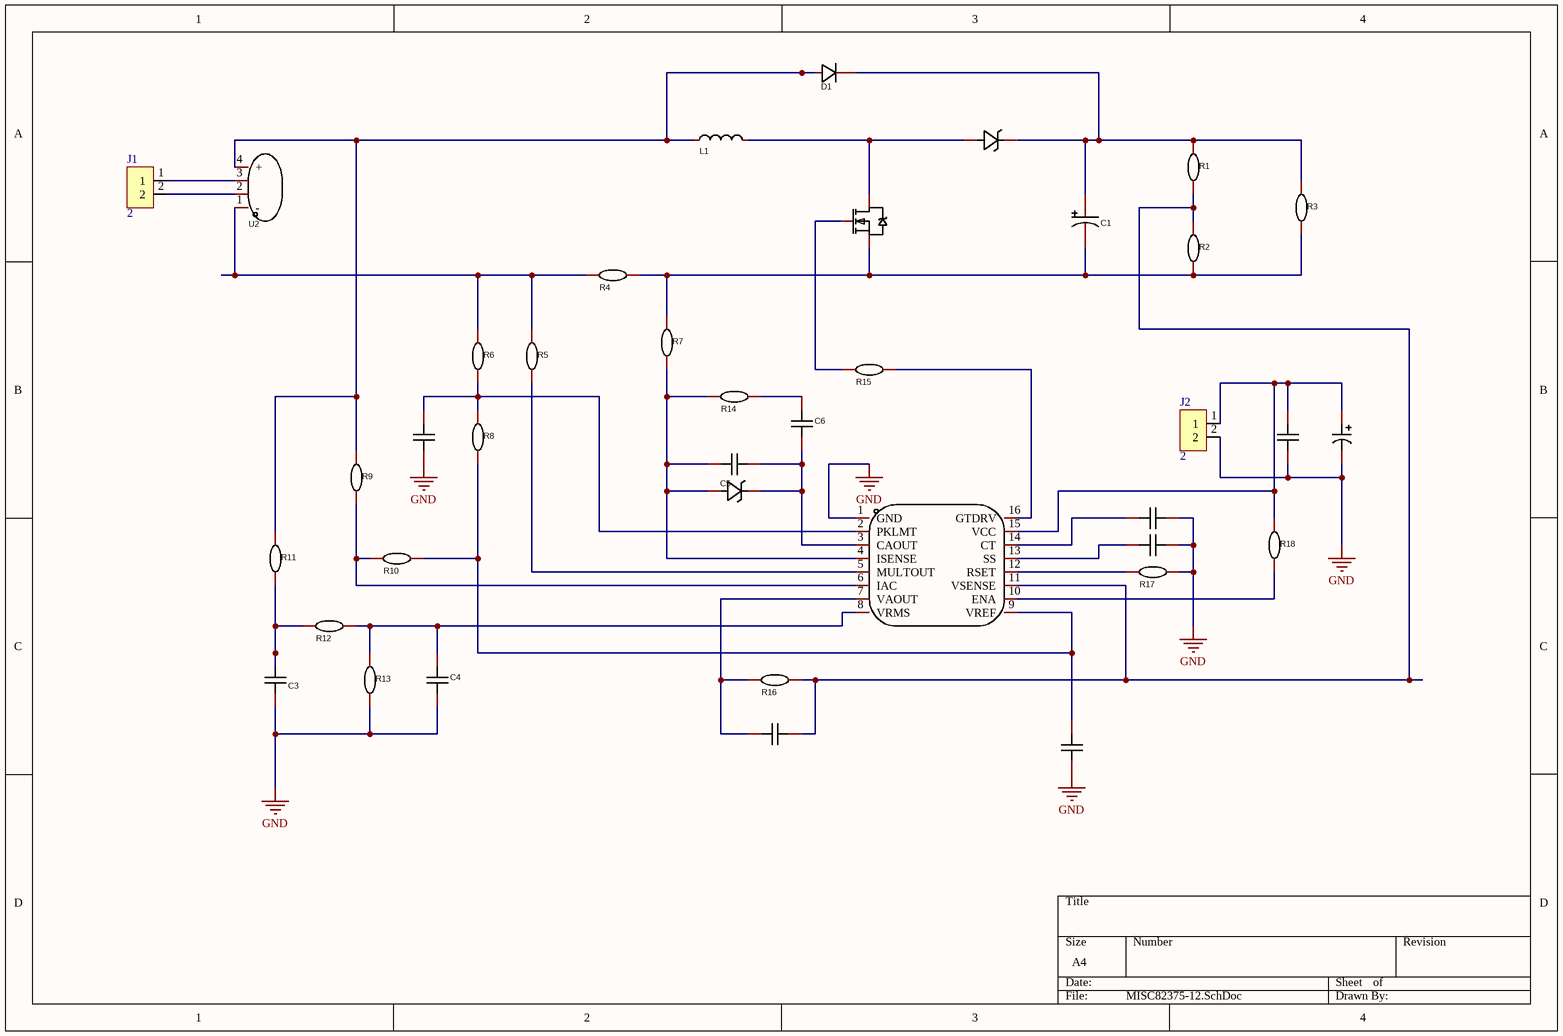
[diagram p0: MISC82375-12.SchDoc]
# Altium project MISC82375-12.PrjPcb
1 sheet, 39 parts. Net scope: global (net labels, ports and power ports of the same name join across sheets).
Board files: MISC82375-2.PcbDoc, MISC82375-4.PcbDoc, MISC82375-6.PcbDoc

## Sheet MISC82375-12.SchDoc
size A4; SheetNumber: 1; SheetTotal: 1

### Parts
C1  LKME1402A101MF  [CAP-TH_BD10.0-P5.00-D1.0-FD]  (value not drawn)
C2  KJKF222M2FF7035A075E  [CAP-TH_L6.5-W3.5-P7.50-D1.0]  (value not drawn)
C3  KY1102M400VAC70Y10093  [CAP-TH_L7.5-W4.5-P10.00-D0.6]  (value not drawn)
C4  CBB21-400V/255JP20  [CAP-TH_L22.0-W12.5-P20.00-D0.7-FD]  (value not drawn)
C5  178MU0002  [CAP-TH_L5.8-W3.6-P5.0-D0.6]  (value not drawn)
C6  178MU0002  [CAP-TH_L5.8-W3.6-P5.0-D0.6]  (value not drawn)
C7  KY1102M400VAC70Y10093  [CAP-TH_L7.5-W4.5-P10.00-D0.6]  (value not drawn)
C8  178MU0002  [CAP-TH_L5.8-W3.6-P5.0-D0.6]  (value not drawn)
C9  178MU0002  [CAP-TH_L5.8-W3.6-P5.0-D0.6]  (value not drawn)
C10  178MU0002  [CAP-TH_L5.8-W3.6-P5.0-D0.6]  (value not drawn)
C11  KY1102M400VAC70Y10093  [CAP-TH_L7.5-W4.5-P10.00-D0.6]  (value not drawn)
C??  RVE100UF35V67RV0072  [CAP-SMD_BD6.3-L6.6-W6.6-LS7.6-FD-1]  (value not drawn)
D1  1N5406_C5338388  [DO-27_BD5.2-L8.9-P12.90-D1.5-RD]  (value not drawn)
D2  GC3D10060A  [TO-220-2_L10.2-W4.5-P5.08-L-A]  (value not drawn)
D3  BZT52C8V2_C19077406  [SOD-123_L2.7-W1.6-LS3.7-RD]  (value not drawn)
J1  2  [DIP2 - duplicate]
J2  2  [DIP2 - duplicate]
L1  XR8*10-101K-L  [IND-TH_BD10.0-P5.00-D0.6]  (value not drawn)
Q1  IRF530NPBF  [TO-220-3_L10.0-W4.5-P2.54-L]  (value not drawn)
R1  MF1/4W-100K±1%-OT26  [RES-TH_BD2.7-L6.2-P10.20-D0.4]  (value not drawn)
R2  MF1/4W-100K±1%-OT26  [RES-TH_BD2.7-L6.2-P10.20-D0.4]  (value not drawn)
R3  MF1/4W-100K±1%-OT26  [RES-TH_BD2.7-L6.2-P10.20-D0.4]  (value not drawn)
R4  MF1/4W-100K±1%-OT26  [RES-TH_BD2.7-L6.2-P10.20-D0.4]  (value not drawn)
R5  MF1/4W-100K±1%-OT26  [RES-TH_BD2.7-L6.2-P10.20-D0.4]  (value not drawn)
R6  MF1/4W-100K±1%-OT26  [RES-TH_BD2.7-L6.2-P10.20-D0.4]  (value not drawn)
R7  MF1/4W-100K±1%-OT26  [RES-TH_BD2.7-L6.2-P10.20-D0.4]  (value not drawn)
R8  MF1/4W-100K±1%-OT26  [RES-TH_BD2.7-L6.2-P10.20-D0.4]  (value not drawn)
R9  MF1/4W-100K±1%-OT26  [RES-TH_BD2.7-L6.2-P10.20-D0.4]  (value not drawn)
R10  MF1/4W-100K±1%-OT26  [RES-TH_BD2.7-L6.2-P10.20-D0.4]  (value not drawn)
R11  MF1/4W-100K±1%-OT26  [RES-TH_BD2.7-L6.2-P10.20-D0.4]  (value not drawn)
R12  MF1/4W-100K±1%-OT26  [RES-TH_BD2.7-L6.2-P10.20-D0.4]  (value not drawn)
R13  MF1/4W-100K±1%-OT26  [RES-TH_BD2.7-L6.2-P10.20-D0.4]  (value not drawn)
R14  MF1/4W-100K±1%-OT26  [RES-TH_BD2.7-L6.2-P10.20-D0.4]  (value not drawn)
R15  MF1/4W-100K±1%-OT26  [RES-TH_BD2.7-L6.2-P10.20-D0.4]  (value not drawn)
R16  MF1/4W-100K±1%-OT26  [RES-TH_BD2.7-L6.2-P10.20-D0.4]  (value not drawn)
R17  MF1/4W-100K±1%-OT26  [RES-TH_BD2.7-L6.2-P10.20-D0.4]  (value not drawn)
R18  MF1/4W-100K±1%-OT26  [RES-TH_BD2.7-L6.2-P10.20-D0.4]  (value not drawn)
U1  UC3854N  [PDIP-16_L19.3-W6.4-P2.54-LS7.94-BL]  (value not drawn)
U2  GBU8K  [GBU_4P-L22.0-W3.5-P5.08-GBU4K]  (value not drawn)

### Nets
GND: C2.1 C3.1 C4.1 C8.1 C9.2 C10.2 C11.1 C??.2 J2.2 R13.1 R17.2 U1.1(GND)
NetC1_1: C1.1 D1.1(C) D2.1(K) R1.2 R3.2
NetC1_2: C1.2 Q1.3(S) R2.1 R3.1 R4.2 R7.2
NetC2_2: C2.2 R6.1 R8.2 U1.2(PKLMT)
NetC3_2: C3.2 R11.1 R12.1
NetC4_2: C4.2 R12.2 R13.2 U1.8(VRMS)
NetC5_1: C5.1 D3.2(A) R7.1 R14.1 U1.4(ISENSE)
NetC5_2: C5.2 C6.1 D3.1(K) U1.3(CAOUT)
NetC6_2: C6.2 R14.2
NetC7_1: C7.1 R16.1 U1.7(VAOUT)
NetC7_2: C7.2 R1.1 R2.2 R16.2 U1.11(VSENSE)
NetC8_2: C8.2 R8.1 R10.2 U1.9(VREF)
NetC9_1: C9.1 U1.13(SS)
NetC10_1: C10.1 U1.14(CT)
NetC11_2: C11.2 C??.1 J2.1 R18.2 U1.15(VCC)
NetD1_2: D1.2(A) L1.1 R9.2 R11.2 U2.4(+)
NetD2_3: D2.3(A) L1.2 Q1.2(D)
NetJ1_1: J1.1 U2.3
NetJ1_2: J1.2 U2.2
NetQ1_1: Q1.1(G) R15.1
NetR4_1: R4.1 R5.2 R6.2 U2.1(-)
NetR5_1: R5.1 U1.5(MULTOUT)
NetR9_1: R9.1 R10.1 U1.6(IAC)
NetR15_2: R15.2 U1.16(GTDRV)
NetR17_1: R17.1 U1.12(RSET)
NetR18_1: R18.1 U1.10(ENA)

### Library data of the parts
C1 = LKME1402A101MF: Manufacturer: Ymin(永铭); Add into BOM: yes; Value: 100uF; Tolerance: ±20%; Rated Voltage: 100V; Ripple Current: 1.04A@100kHz; φD: 10mm; L: 14mm; Lifetime @ Temp: 10000hrs@105℃; Symbol: LKME1402A101MF; Device: LKME1402A101MF; LCSC Part Name: 100uF ±20% 100V; Supplier Part: C443138; Manufacturer Part: LKME1402A101MF; Supplier Footprint: 插件,D10xL14mm; JLCPCB Part Class: Extended Part; Datasheet: https://atta.szlcsc.com/upload/public/pdf/source/20200220/C487520_443A40905984A455D375EE990FEAA9E8.pdf; Supplier: LCSC; Convert to PCB: yes; Equivalent Series Resistance(ESR): -; Lead Spacing: 5mm
C2 = KJKF222M2FF7035A075E: Manufacturer: KNSCHA(科尼盛); Add into BOM: yes; Value: 2.2nF; Tolerance: ±20%; Voltage(AC): 300V; Subclass: Y2; safety certification: UL; ENEC; VDE; CQC; Symbol: KJKF222M2FF7035A075E; Device: KJKF222M2FF7035A075E; LCSC Part Name: 2.2nF ±20% 300V 等级:Y2; Supplier Part: C2803195; Manufacturer Part: KJKF222M2FF7035A075E; Supplier Footprint: 插件,P=7.5mm; JLCPCB Part Class: Extended Part; Datasheet: https://atta.szlcsc.com/upload/public/pdf/source/20210420/C2803195_BA0DBC8778A43A5602C5594119034AD5.pdf; Supplier: LCSC; Convert to PCB: yes
C3 C7 C11 = KY1102M400VAC70Y10093: Manufacturer: KNSCHA(科尼盛); Value: 1nF; Add into BOM: yes; Tolerance: ±20%; Voltage(AC): 400V; Subclass: Y1; safety certification: UL; ENEC; VDE; CQC; Symbol: KY1102M400VAC70Y10093; Device: KY1102M400VAC70Y10093; Supplier: LCSC; Supplier Part: C2943996; Manufacturer Part: KY1102M400VAC70Y10093; JLCPCB Part Class: Extended Part; LCSC Part Name: 1nF ±20% 400V 等级:Y1; Supplier Footprint: 插件,P=10mm; Datasheet: https://atta.szlcsc.com/upload/public/pdf/source/20220125/2D2B80E2C5D988A5B116EA64517B63EA.pdf; Convert to PCB: yes
C4 = CBB21-400V/255JP20: Manufacturer: 东通电子; Add into BOM: yes; Value: 2.5uF; Tolerance: ±5%; Voltage Rated: 400V; Symbol: CBB21-400V/255JP20; Device: CBB21-400V/255JP20; LCSC Part Name: 2.5uF ±5% 400V; Supplier Part: C2913178; Manufacturer Part: CBB21-400V/255JP20; Supplier Footprint: 插件,P=20mm; JLCPCB Part Class: Extended Part; Datasheet: https://atta.szlcsc.com/upload/public/pdf/source/20211116/A54D0E5F37ACF7C4504A98327CA0E134.pdf; Supplier: LCSC; Convert to PCB: yes
C5 C6 C8-C10 = 178MU0002: Manufacturer: KNSCHA(科尼盛); Value: 100nF; Add into BOM: yes; Tolerance: ±10%; Voltage Rated: 50V; Temperature Coefficient: X7R; Symbol: 178MU0002; Device: 178MU0002; Supplier: LCSC; Supplier Part: C5632426; Manufacturer Part: 178MU0002; JLCPCB Part Class: Extended Part; LCSC Part Name: 100nF ±10% 50V; Supplier Footprint: 插件,P=5.08mm; Datasheet: https://atta.szlcsc.com/upload/public/pdf/source/20230506/08E784E6BF236BA57EBA91152AC3AC6D.pdf; Convert to PCB: yes
C?? = RVE100UF35V67RV0072: Manufacturer: KNSCHA(科尼盛); Add into BOM: yes; Value: 100uF; Tolerance: ±20%; Rated Voltage: 35V; Ripple Current: 230mA@120Hz; Equivalent Series Resistance(ESR): 600mΩ@100kHz; φD: 6.3mm; L: 7.7mm; Lifetime @ Temp: 2000hrs@105℃; Symbol: RVE100UF35V67RV0072; Device: RVE100UF35V67RV0072; LCSC Part Name: 100uF ±20% 35V; Supplier Part: C2836437; Manufacturer Part: RVE100UF35V67RV0072; Supplier Footprint: SMD,D6.3xL7.7mm; JLCPCB Part Class: Extended Part; Datasheet: https://atta.szlcsc.com/upload/public/pdf/source/20220719/B52EB46F8A1558448ED03D8B4CB3C24F.pdf; Supplier: LCSC; Convert to PCB: yes; Operating Temperature: -55℃~+105℃
D1 = 1N5406_C5338388: Manufacturer: SUNMATE(森美特); Manufacturer Part: 1N5406; Add into BOM: yes; Forward Voltage (Vf@If): 1V@3A; Reverse Voltage (Vr): 600V; Average Rectified Current (Io): 3A; Reverse Leakage Current: 10uA@600V; Symbol: 1N5406_C5338388; Device: 1N5406_C5338388; LCSC Part Name: 电压:600V 电流:3A; Supplier Part: C5338388; Supplier Footprint: DO-27; Datasheet: https://atta.szlcsc.com/upload/public/pdf/source/20221227/E8B5F2A8C1FD9CCCBF5FF47F6842D4A3.pdf; Supplier: LCSC; Convert to PCB: yes
D2 = GC3D10060A: Manufacturer: SUPSiC(国晶微半导体); Add into BOM: yes; Average Rectified Current (Io): 30A; Forward Voltage (Vf@If): 1.5V; Reverse Voltage (Vr): 600V; Symbol: GC3D10060A; Device: GC3D10060A; LCSC Part Name: GC3D10060A; Supplier Part: C7435067; Manufacturer Part: GC3D10060A; Supplier Footprint: TO-220-2; Datasheet: https://atta.szlcsc.com/upload/public/pdf/source/20230905/31DB1507024993D4A9FE1C88E19B495D.pdf; Supplier: LCSC; Convert to PCB: yes
D3 = BZT52C8V2_C19077406: Manufacturer: 宏迦橙; Add into BOM: yes; Diode Configuration: parameter Diode Configuration Single; Zener Voltage (Nom): 8.2V; Reverse Leakage Current (Ir): 700nA@5V; Zener Voltage (Range): 7.79V~8.61V; Power Dissipation: 500mW; Zener Impedance (Zzt): 15Ω; Symbol: BZT52C8V2_C19077406; Device: BZT52C8V2_C19077406; Supplier: LCSC; Supplier Part: C19077406; Manufacturer Part: BZT52C8V2; LCSC Part Name: BZT52C8V2; Supplier Footprint: SOD-123; Datasheet: https://atta.szlcsc.com/upload/public/pdf/source/20231117/6E01C14CCA1A38C68A5225952E4BCE14.pdf; Convert to PCB: yes
J1 J2 = AC_in
L1 = XR8*10-101K-L: Manufacturer: XR(祥如); Add into BOM: yes; Value: 100uH; Tolerance: ±10%; Type: parameter Type text I-type inductor; Symbol: XR8*10-101K-L; Device: XR8*10-101K-L; LCSC Part Name: 100uH ±10% 工字电感; Supplier Part: C5380241; Manufacturer Part: XR8*10-101K-L; Supplier Footprint: 插件,D8xL10mm; JLCPCB Part Class: Extended Part; Datasheet: https://atta.szlcsc.com/upload/public/pdf/source/20230323/E8473EC4B67CAA12E996DDE863677D9C.pdf; Supplier: LCSC; Convert to PCB: yes
Q1 = IRF530NPBF: Manufacturer: Infineon(英飞凌); Add into BOM: yes; Type: parameter Type text N-channel; Drain Source Voltage (Vdss): 100V; Continuous Drain Current (Id): 17A; Power Dissipation (Pd): 70W; Drain Source On Resistance (RDS(on)@Vgs,Id): 90mΩ@10V,9A; Gate Threshold Voltage (Vgs(th)@Id): 4V@250uA; Total Gate Charge (Qg@Vgs): 37nC@10V; Input Capacitance (Ciss@Vds): 920pF@25V; Symbol: IRF530NPBF; Device: IRF530NPBF; LCSC Part Name: N沟道 耐压:100V 电流:17A; Supplier Part: C2565; Manufacturer Part: IRF530NPBF; Supplier Footprint: TO-220AB; JLCPCB Part Class: Extended Part; Datasheet: https://atta.szlcsc.com/upload/public/pdf/source/20200421/C513195_D9CEFFCD00D3D7736B96C248E8CC28A6.pdf; Supplier: LCSC; Convert to PCB: yes; Operating Temperature: -55℃~+175℃@(Tj)
R1-R18 = MF1/4W-100K±1%-OT26: Manufacturer: VO(翔胜); Value: 100kΩ; Add into BOM: yes; Tolerance: ±1%; Overload Voltage (Max): 250V; Power(Watts): 250mW; Temperature Coefficient: ±350ppm/℃; Symbol: MF1/4W-100K±1%-OT26; Device: MF1/4W-100K±1%-OT26; Supplier: LCSC; Supplier Part: C2843019; Manufacturer Part: MF1/4W-100K±1%-OT26; JLCPCB Part Class: Extended Part; LCSC Part Name: 金属膜电阻 100kΩ ±1% 250mW; Supplier Footprint: 插件,2.7x6.2mm; Datasheet: https://atta.szlcsc.com/upload/public/pdf/source/20200609/C601728_5AA4C0C8E12E11069DA2C3356F29D1F2.pdf; Convert to PCB: yes; Type: parameter Type text Metal film resistor; Operating Temperature Range: -55℃~+155℃
U1 = UC3854N: Manufacturer: TI(德州仪器); Add into BOM: yes; Supply Voltage: 14.5V~30V; Switching Frequency: 200kHz; Symbol: UC3854N; Device: UC3854N; LCSC Part Name: UC3854N; Supplier Part: C2867379; Manufacturer Part: UC3854N; Supplier Footprint: PDIP-16; JLCPCB Part Class: Extended Part; Datasheet: https://www.ti.com/cn/lit/gpn/uc2854; Supplier: LCSC; Convert to PCB: yes; Operating Temperature: 0℃~+70℃
U2 = GBU8K: Manufacturer: LRC(乐山无线电); Symbol: GBU8K_C383156; Add into BOM: yes; Forward Voltage (Vf@If): 1.1V; Reverse Voltage (Vr): 800V; Average Rectified Current (Io): 8A; Reverse Leakage Current (Ir): 5uA; Peak Forward Surge Current: 175A; Device: GBU8K; Supplier: LCSC; Supplier Part: C383156; Manufacturer Part: GBU8K; JLCPCB Part Class: Extended Part; LCSC Part Name: 电压:800V 电流:8A; Supplier Footprint: GBU; Datasheet: https://atta.szlcsc.com/upload/public/pdf/source/20211216/BBDE0A70898025107B56F4C05CE90C86.pdf; Convert to PCB: yes; Operating Temperature: -55℃~+150℃@(Tj)